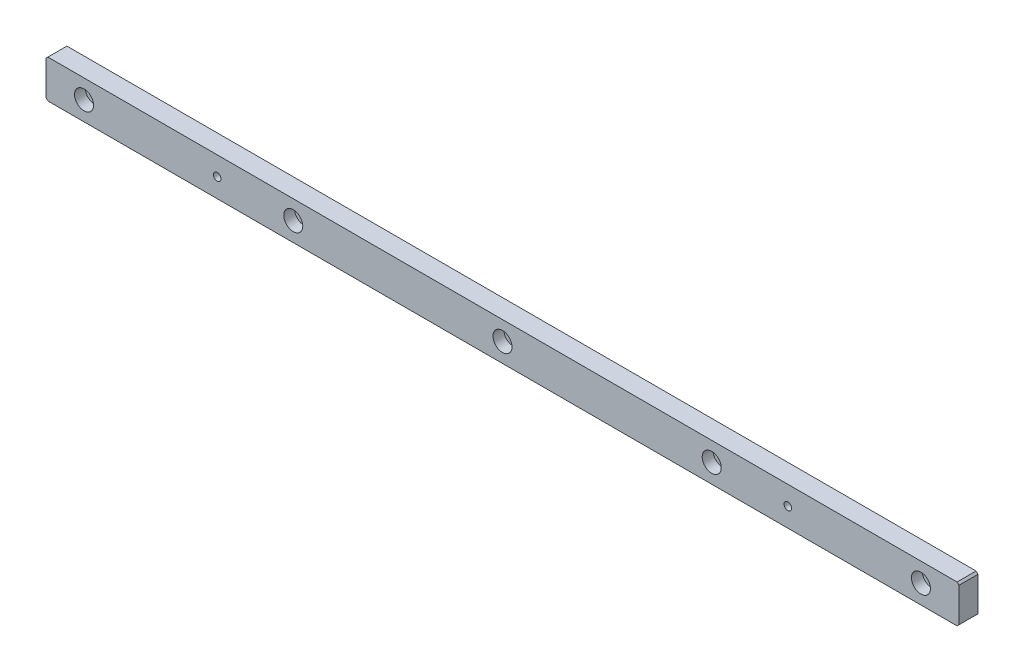
from build123d import *

# Parameters (mm, degrees)
SKETCH1_W                                            = 480
SKETCH1_H                                            = 20
BOSS_EXTRUDE1_DEPTH                                  = 10
HOLE_SIZE_PER_SOCKET_HEAD_CAP_SCREW_TYPE_D           = 5.5
HOLE_SIZE_PER_SOCKET_HEAD_CAP_SCREW_TYPE_CBORE_D     = 10
HOLE_SIZE_PER_SOCKET_HEAD_CAP_SCREW_TYPE_CBORE_DEPTH = 5.7
CHAMFER1_SIZE                                        = 1
F_4_0_4_DIAMETER_HOLE1_D                             = 4
F_4_0_4_DIAMETER_HOLE1_DEPTH                         = 12
F_4_0_4_DIAMETER_HOLE1_TIP                           = 1.201721238


with BuildPart() as part:
    # Sketch1 → Boss-Extrude1 (new body)
    with BuildSketch(Plane.XY):
        Rectangle(SKETCH1_W, SKETCH1_H)
    extrude(amount=BOSS_EXTRUDE1_DEPTH)

    # Hole size per socket head cap screw type1 (through all)
    with Locations(Plane.XY.offset(10)):
        with Locations((0, 0), (-110, 0), (110, 0), (220, 0), (-220, 0)):
            CounterBoreHole(HOLE_SIZE_PER_SOCKET_HEAD_CAP_SCREW_TYPE_D / 2, HOLE_SIZE_PER_SOCKET_HEAD_CAP_SCREW_TYPE_CBORE_D / 2, HOLE_SIZE_PER_SOCKET_HEAD_CAP_SCREW_TYPE_CBORE_DEPTH)

    # Chamfer1
    chamfer1_edges = [part.edges().sort_by_distance(p)[0] for p in [
        (240, -10, 5),
        (-240, -10, 5),
        (-240, 10, 5),
        (240, 10, 5),
    ]]
    chamfer(chamfer1_edges, length=CHAMFER1_SIZE)

    # Ø4.0 (4) Diameter Hole1
    with Locations(Plane.XY.offset(10)):
        with Locations((-150, 0), (150, 0)):
            Hole(F_4_0_4_DIAMETER_HOLE1_D / 2, depth=F_4_0_4_DIAMETER_HOLE1_DEPTH)
            with Locations((0, 0, -(F_4_0_4_DIAMETER_HOLE1_DEPTH + F_4_0_4_DIAMETER_HOLE1_TIP / 2))):  # 118° drill point
                Cone(0, F_4_0_4_DIAMETER_HOLE1_D / 2, F_4_0_4_DIAMETER_HOLE1_TIP, mode=Mode.SUBTRACT)


solid = part.part
